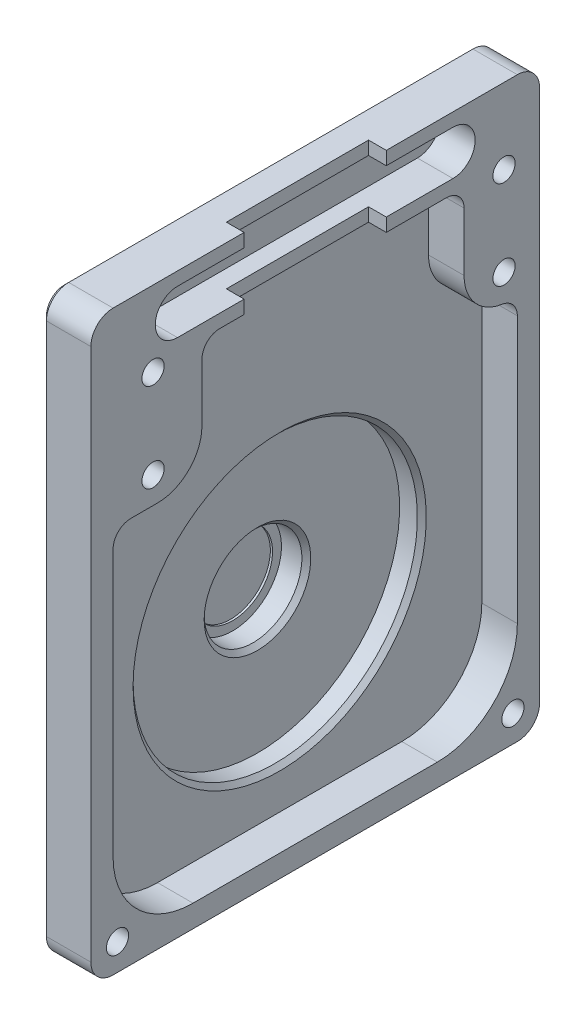
from build123d import *

# Parameters (mm, degrees)
SKETCH_1_W          = 101
SKETCH_1_H          = 130
EXTRUDE_1_DEPTH     = 11
CUT_EXTRUDE_1_DEPTH = 8
CUT_EXTRUDE_2_DEPTH = 8
CUT_EXTRUDE_3_REACH = 1271.625
SKETCH_4_W          = 4
SKETCH_4_H          = 32
CUT_EXTRUDE_4_REACH = 1273.161
SKETCH_5_W          = 4
SKETCH_5_H          = 32
SKETCH_6_R          = 36
EXTRUDE_2_DEPTH     = 5
SKETCH_7_R          = 14
EXTRUDE_3_DEPTH     = 4.5
SKETCH_8_R          = 32
CUT_EXTRUDE_5_DEPTH = 5
SKETCH_9_R          = 11
CUT_EXTRUDE_6_DEPTH = 5.6
SKETCH_10_R         = 9
CUT_EXTRUDE_7_DEPTH = 0.5
HOLE_WIZARD_M6_1_D  = 5
FILLET_1_R          = 5
CHAMFER_1_SIZE      = 1
FILLET_2_R          = 2
FILLET_3_R          = 4
FILLET_4_R          = 10


with BuildPart() as part:
    # 草图1 → 凸台-拉伸1 (new body)
    with BuildSketch(Plane(origin=(1263, 0, 0), x_dir=(0, 0, -1), z_dir=(1, 0, 0))):
        with Locations((11, -6.6)):
            Rectangle(SKETCH_1_W, SKETCH_1_H)
    extrude(amount=-EXTRUDE_1_DEPTH)

    # 草图2 → 切除-拉伸1 (cut)
    with BuildSketch(Plane(origin=(1263, 0, 0), x_dir=(0, 0, -1), z_dir=(1, 0, 0))):
        with BuildLine():
            Line((44.5, 25.256406461), (44.5, 42.4))
            Line((44.5, 42.4), (-14.5, 42.4))
            Line((-14.5, 42.4), (-14.5, 15.4))
            Line((-14.5, 15.4), (-34.5, 15.4))
            Line((-34.5, 15.4), (-34.5, -48.6))
            ThreePointArc((-34.5, -48.6), (-29.227922061, -61.327922061), (-16.5, -66.6))
            Line((-16.5, -66.6), (38.5, -66.6))
            ThreePointArc((38.5, -66.6), (51.227922061, -61.327922061), (56.5, -48.6))
            Line((56.5, -48.6), (56.5, 15.458447489))
            ThreePointArc((56.5, 15.458447489), (48.17544468, 17.510439768), (44.5, 25.256406461))
        make_face()
    extrude(amount=-CUT_EXTRUDE_1_DEPTH, mode=Mode.SUBTRACT)

    # 草图3 → 切除-拉伸2 (cut)
    with BuildSketch(Plane(origin=(1263, 0, 0), x_dir=(0, 0, -1), z_dir=(1, 0, 0))):
        with BuildLine():
            Line((42, 55.4), (-20, 55.4))
            ThreePointArc((-20, 55.4), (-25, 50.4), (-20, 45.4))
            Line((-20, 45.4), (42, 45.4))
            ThreePointArc((42, 45.4), (47, 50.4), (42, 55.4))
        make_face()
    extrude(amount=-CUT_EXTRUDE_2_DEPTH, mode=Mode.SUBTRACT)

    # 草图4 → 切除-拉伸3 (cut, up to next)
    with BuildSketch(Plane.XZ.offset(-42.4), mode=Mode.PRIVATE) as cut_extrude_3_sk1:
        with Locations((1261, -11)):
            Rectangle(SKETCH_4_W, SKETCH_4_H)
    cut_extrude_3_tool1 = extrude(cut_extrude_3_sk1.sketch, amount=-CUT_EXTRUDE_3_REACH, mode=Mode.PRIVATE) & part.part
    add(cut_extrude_3_tool1.solids().sort_by_distance((1261, 42.4, -11))[0], mode=Mode.SUBTRACT)

    # 草图5 → 切除-拉伸4 (cut, up to next)
    with BuildSketch(Plane(origin=(0, 58.4, 0), x_dir=(-1, 0, 0), z_dir=(0, 1, 0)), mode=Mode.PRIVATE) as cut_extrude_4_sk1:
        with Locations((-1261, -11)):
            Rectangle(SKETCH_5_W, SKETCH_5_H)
    cut_extrude_4_tool1 = extrude(cut_extrude_4_sk1.sketch, amount=-CUT_EXTRUDE_4_REACH, mode=Mode.PRIVATE) & part.part
    add(cut_extrude_4_tool1.solids().sort_by_distance((1261, 58.4, -11))[0], mode=Mode.SUBTRACT)

    # 草图6 → 凸台-拉伸2 (add)
    with BuildSketch(Plane.ZY.offset(-1252)):
        with Locations((-11, -25.6)):
            Circle(SKETCH_6_R)
    extrude(amount=EXTRUDE_2_DEPTH)

    # 草图7 → 凸台-拉伸3 (add)
    with BuildSketch(Plane.ZY.offset(-1247)):
        with Locations(Location((-11, -25.6, 0), (0, 0, 180))):
            Circle(SKETCH_7_R)
    extrude(amount=EXTRUDE_3_DEPTH)

    # 草图8 → 切除-拉伸5 (cut)
    with BuildSketch(Plane(origin=(1255, 0, 0), x_dir=(0, 0, -1), z_dir=(1, 0, 0))):
        with Locations(Location((11, -25.6, 0), (0, 0, 180))):
            Circle(SKETCH_8_R)
    extrude(amount=-CUT_EXTRUDE_5_DEPTH, mode=Mode.SUBTRACT)

    # 草图9 → 切除-拉伸6 (cut)
    with BuildSketch(Plane(origin=(1250, 0, 0), x_dir=(0, 0, -1), z_dir=(1, 0, 0))):
        with Locations(Location((11, -25.6, 0), (0, 0, 180))):
            Circle(SKETCH_9_R)
    extrude(amount=-CUT_EXTRUDE_6_DEPTH, mode=Mode.SUBTRACT)

    # 草图10 → 切除-拉伸7 (cut)
    with BuildSketch(Plane(origin=(1244.4, 0, 0), x_dir=(0, 0, -1), z_dir=(1, 0, 0))):
        with Locations(Location((11, -25.6, 0), (0, 0, 180))):
            Circle(SKETCH_10_R)
    extrude(amount=-CUT_EXTRUDE_7_DEPTH, mode=Mode.SUBTRACT)

    # M6 螺纹孔1 (through all)
    with Locations(Plane(origin=(1263, 0, 0), x_dir=(0, 0, -1), z_dir=(1, 0, 0))):
        with Locations((53.5, 41.4), (-25.5, 41.4), (-25.5, 21.4), (-33.5, -65.6), (55.5, -65.6), (53.5, 21.4)):
            Hole(HOLE_WIZARD_M6_1_D / 2)

    # 圆角1
    fillet_1_edges = [part.edges().sort_by_distance(p)[0] for p in [
        (1257.5, -71.6, 39.5),
        (1257.5, 58.4, 39.5),
        (1257.5, 58.4, -61.5),
        (1257.5, -71.6, -61.5),
    ]]
    fillet(fillet_1_edges, radius=FILLET_1_R)

    # 倒角1
    chamfer_1_edges = [part.edges().sort_by_distance(p)[0] for p in [
        (1252, -6.6, -61.5),
        (1252, 58.4, -11),
        (1252, -71.6, -11),
        (1252, -6.6, 39.5),
        (1252, -70.135533906, 38.035533906),
        (1252, 56.935533906, 38.035533906),
        (1252, -70.135533906, -60.035533906),
        (1252, 56.935533906, -60.035533906),
        (1255, -25.6, -43),
        (1250, -25.6, -22),
    ]]
    chamfer(chamfer_1_edges, length=CHAMFER_1_SIZE)

    # 圆角2
    fillet_2_edges = [part.edges().sort_by_distance(p)[0] for p in [
        (1252, -25.6, -47),
        (1247, -25.6, -47),
        (1247, -25.6, 3),
        (1242.5, -25.6, 3),
    ]]
    fillet(fillet_2_edges, radius=FILLET_2_R)

    # 圆角3
    fillet_3_edges = [part.edges().sort_by_distance(p)[0] for p in [
        (1259, 15.458447489, -56.5),
        (1259, 15.4, 34.5),
        (1259, 42.4, 14.5),
        (1259, 42.4, -44.5),
    ]]
    fillet(fillet_3_edges, radius=FILLET_3_R)

    # 圆角4
    fillet_4_edges = [part.edges().sort_by_distance(p)[0] for p in [
        (1259, 15.4, 14.5),
    ]]
    fillet(fillet_4_edges, radius=FILLET_4_R)


solid = part.part
